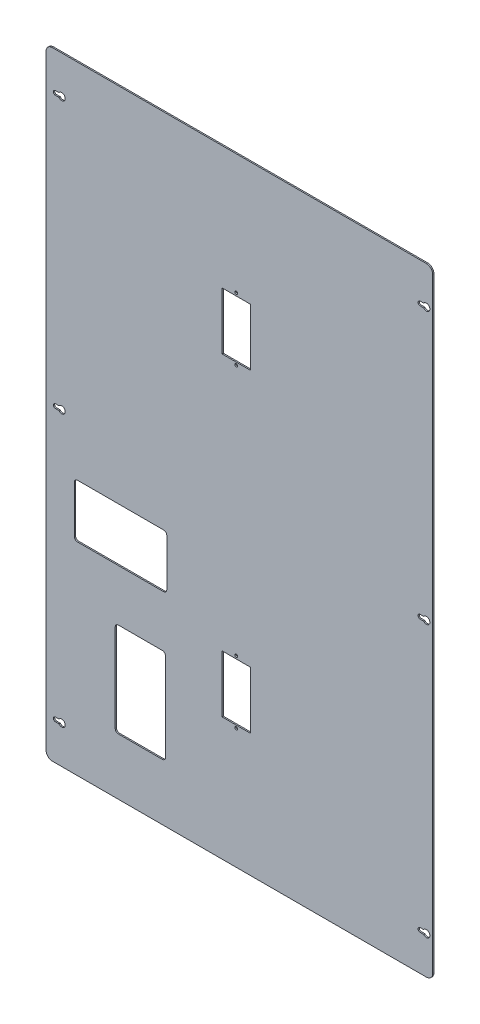
SolidWorks part; units mm, degrees
material "SPCC"
ref_plane "Front Plane" through (0, 0, 0) normal (0, 0, 1) x (1, 0, 0)
ref_plane "Top Plane" through (0, 0, 0) normal (0, 1, 0) x (1, 0, 0)
ref_plane "Right Plane" through (0, 0, 0) normal (1, 0, 0) x (0, 0, -1)
sketch "Sketch1" plane through (0, 0, 0) normal (0, 0, 1) x (1, 0, 0)
  line L1 (-307.5, 491.5) -> (307.5, 491.5)
  line L2 (-307.5, 491.5) -> (-307.5, -491.5)
  line L3 (-307.5, -491.5) -> (307.5, -491.5)
  line L4 (307.5, 491.5) -> (307.5, -491.5)
  line L5 (-307.5, 491.5) -> (307.5, -491.5) construction
  line L6 (-307.5, -491.5) -> (307.5, 491.5) construction
  point P0 (0, 0)
  dimension "D1" = 615
  dimension "D2" = 983
extrude "Boss-Extrude1" add sketch "Sketch1" along normal blind 2
sketch "Sketch7" plane through (0, 0, 0) normal (0, 0, -1) x (-1, 0, 0)
  line L1 (-17.5, 295.5) -> (27.5, 295.5)
  line L2 (-17.5, 295.5) -> (-17.5, 204.5)
  line L3 (-17.5, 204.5) -> (27.5, 204.5)
  line L4 (27.5, 295.5) -> (27.5, 204.5)
  line L5 (-17.5, 295.5) -> (27.5, 204.5) construction
  line L6 (-17.5, 204.5) -> (27.5, 295.5) construction
  line L7 (-17.5, -204.5) -> (27.5, -204.5)
  line L8 (-17.5, -204.5) -> (-17.5, -295.5)
  line L9 (-17.5, -295.5) -> (27.5, -295.5)
  line L10 (27.5, -204.5) -> (27.5, -295.5)
  line L11 (-17.5, -204.5) -> (27.5, -295.5) construction
  line L12 (-17.5, -295.5) -> (27.5, -204.5) construction
  point P0 (5, 250)
  point P5 (5, -250)
  dimension "D1" = 5
  dimension "D2" = 91
  dimension "D3" = 45
  dimension "D4" = 250
  dimension "D5" = 250
extrude "Cut-Extrude4" cut sketch "Sketch7" against normal through all
sketch "Sketch8" plane through (0, 0, 0) normal (0, 0, -1) x (-1, 0, 0)
  line L0 (5, -295.5) -> (5, -204.5) construction
  line L1 (-17.5, -295.5) -> (27.5, -295.5) construction
  line L2 (27.5, -204.5) -> (-17.5, -204.5) construction
  line L3 (-17.5, 204.5) -> (27.5, 204.5) construction
  circle A0 centre (5, 300) radius 2.25
  circle A1 centre (5, 200) radius 2.25
  circle A2 centre (5, -200) radius 2.25
  circle A3 centre (5, -300) radius 2.25
  dimension "D1" = 100
  dimension "D2" = 4.5
  dimension "D3" = 4.5
  dimension "D4" = 100
  dimension "D5" = 4.5
extrude "Cut-Extrude5" cut sketch "Sketch8" against normal through all
fillet "Fillet3" radius 10 4 edges at (307.5, -491.5, 1) (307.5, 491.5, 1) (-307.5, 491.5, 1) (-307.5, -491.5, 1)
sketch "Sketch10" plane through (0, 0, 0) normal (0, 0, -1) x (-1, 0, 0)
  line L0 (-297.5, 491.5) -> (297.5, 491.5) construction
  line L1 (307.5, 481.5) -> (307.5, -481.5) construction
  line L2 (292.5, 434.8) -> (286.9, 434.8)
  line L3 (292.5, 428.2) -> (286.9, 428.2)
  arc A0 (292.5, 428.2) -> (292.5, 434.8) centre (292.5, 431.5) ccw
  arc A1 (286.9, 434.8) -> (286.9, 428.2) centre (282.5, 431.5) ccw
  dimension "D4" = 11
  dimension "D5" = 6.6
  dimension "D1" = 60
  dimension "D2" = 15
  dimension "D3" = 10
extrude "Cut-Extrude6" cut sketch "Sketch10" against normal blind 10
pattern_linear "LPattern1" count 3 spacing 431.5 along (0, -1, 0) count 2 spacing 580 along (1, 0, 0) of "Cut-Extrude6"
sketch "Sketch11" plane through (0, 0, 2) normal (0, 0, 1) x (1, 0, 0)
  line L0 (-297.5, -491.5) -> (297.5, -491.5) construction
  line L1 (97.5, 518.5) -> (247.5, 518.5)
  line L2 (97.5, 518.5) -> (97.5, 268.5)
  line L3 (97.5, 268.5) -> (247.5, 268.5)
  line L4 (247.5, 518.5) -> (247.5, 268.5)
  line L5 (97.5, -181.5) -> (247.5, -181.5)
  line L6 (97.5, -181.5) -> (97.5, -411.5)
  line L7 (97.5, -411.5) -> (247.5, -411.5)
  line L8 (247.5, -181.5) -> (247.5, -411.5)
  line L9 (307.5, -481.5) -> (307.5, 481.5) construction
  dimension "D1" = 80
  dimension "D2" = 230
  dimension "D3" = 450
  dimension "D4" = 250
  dimension "D5" = 60
  dimension "D6" = 150
extrude "Cut-Extrude7" [suppressed] cut sketch "Sketch11" against normal through all
sketch "Sketch12" plane through (0, 0, 2) normal (0, 0, 1) x (1, 0, 0)
  line L1 (-197.5, -251.5) -> (-117.5, -251.5)
  line L2 (-197.5, -251.5) -> (-197.5, -401.5)
  line L3 (-197.5, -401.5) -> (-117.5, -401.5)
  line L4 (-117.5, -251.5) -> (-117.5, -401.5)
  line L5 (-307.5, 481.5) -> (-307.5, -481.5) construction
  line L6 (-297.5, -491.5) -> (297.5, -491.5) construction
  dimension "D1" = 90
  dimension "D2" = 150
  dimension "D3" = 110
  dimension "D4" = 80
extrude "Cut-Extrude8" cut sketch "Sketch12" against normal through all
sketch "Sketch13" plane through (0, 0, 0) normal (0, 0, -1) x (-1, 0, 0)
  line L0 (307.5, 481.5) -> (307.5, -481.5) construction
  line L1 (115.5, -84.5) -> (262.5, -84.5)
  line L2 (115.5, -84.5) -> (115.5, -169.5)
  line L3 (115.5, -169.5) -> (262.5, -169.5)
  line L4 (262.5, -84.5) -> (262.5, -169.5)
  line L5 (117.5, -251.5) -> (197.5, -251.5) construction
  dimension "D1" = 45
  dimension "D2" = 85
  dimension "D3" = 147
  dimension "D4" = 82
extrude "Cut-Extrude9" cut sketch "Sketch13" against normal blind 10
fillet "Fillet4" radius 5 8 edges at (-117.5, -401.5, 1) (-197.5, -401.5, 1) (-197.5, -251.5, 1) (-117.5, -251.5, 1) (-115.5, -84.5, 1) (-115.5, -169.5, 1) (-262.5, -169.5, 1) (-262.5, -84.5, 1)
